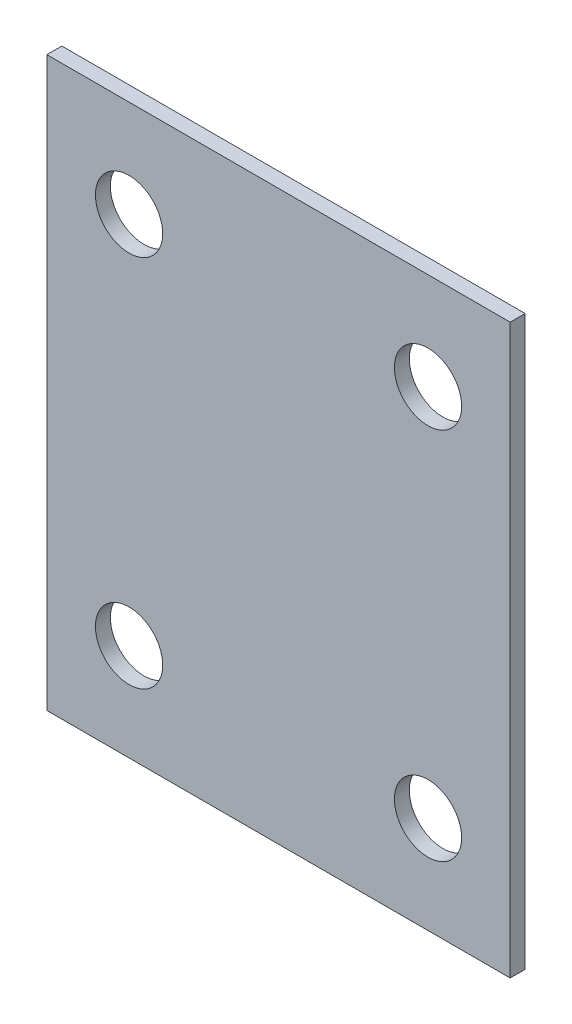
SolidWorks part; units mm, degrees
ref_plane "前视基准面" through (0, 0, 0) normal (0, 0, 1) x (1, 0, 0)
ref_plane "上视基准面" through (0, 0, 0) normal (0, 1, 0) x (1, 0, 0)
ref_plane "右视基准面" through (0, 0, 0) normal (1, 0, 0) x (0, 0, -1)
sketch "草图1" plane through (0, 0, 0) normal (0, 0, 1) x (1, 0, 0)
  line L1 (15.5, -19) -> (-15.5, -19)
  line L2 (15.5, -19) -> (15.5, 19)
  line L3 (15.5, 19) -> (-15.5, 19)
  line L4 (-15.5, -19) -> (-15.5, 19)
  line L5 (15.5, -19) -> (-15.5, 19) construction
  line L6 (15.5, 19) -> (-15.5, -19) construction
  line L7 (10, -12.5) -> (-10, -12.5) construction
  line L8 (10, -12.5) -> (10, 12.5) construction
  line L9 (10, 12.5) -> (-10, 12.5) construction
  line L10 (-10, -12.5) -> (-10, 12.5) construction
  line L11 (10, -12.5) -> (-10, 12.5) construction
  line L12 (10, 12.5) -> (-10, -12.5) construction
  circle A0 centre (-10, 12.5) radius 2.25
  circle A1 centre (10, 12.5) radius 2.25
  circle A2 centre (10, -12.5) radius 2.25
  circle A3 centre (-10, -12.5) radius 2.25
  point P0 (0, 0)
  point P5 (0, 0)
  dimension "D5" = 4.5
  dimension "D1" = 31
  dimension "D2" = 38
  dimension "D3" = 20
  dimension "D4" = 25
extrude "凸台-拉伸1" add sketch "草图1" along normal blind 1
